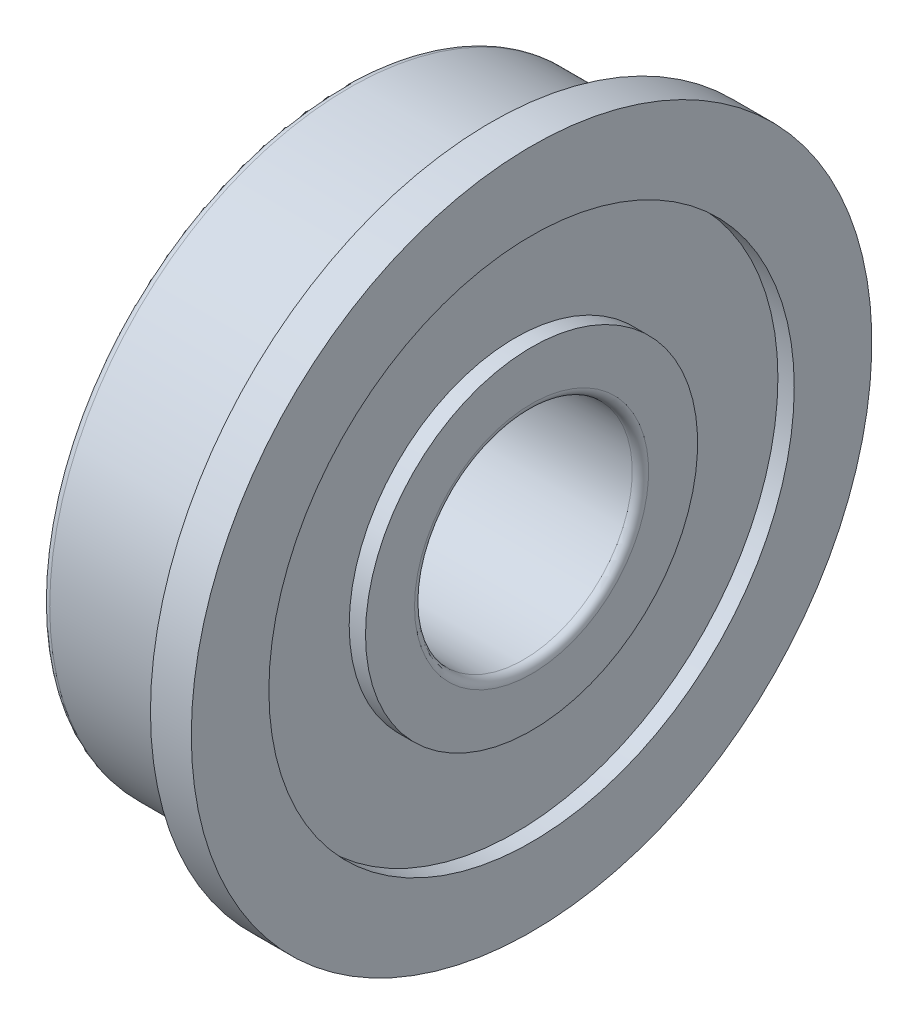
from build123d import *


with BuildPart() as part:
    # Sketch1 → Revolve1 (revolve)
    with BuildSketch(Plane.XY, mode=Mode.PRIVATE) as revolve1_sk:
        with BuildLine():
            Line((0, 10.7), (0, 9.65))
            Line((0, 9.65), (0.6, 9.65))
            Line((0.6, 9.65), (0.6, 6.1))
            Line((0.6, 6.1), (0, 6.1))
            Line((0, 6.1), (0, 4.3))
            ThreePointArc((0, 4.3), (0.087867966, 4.087867966), (0.3, 4))
            Line((0.3, 4), (6.7, 4))
            ThreePointArc((6.7, 4), (6.912132034, 4.087867966), (7, 4.3))
            Line((7, 4.3), (7, 6.1))
            Line((7, 6.1), (6.4, 6.1))
            Line((6.4, 6.1), (6.4, 9.65))
            Line((6.4, 9.65), (7, 9.65))
            Line((7, 9.65), (7, 12.5))
            Line((7, 12.5), (5.5, 12.5))
            Line((5.5, 12.5), (5.5, 11.3))
            ThreePointArc((5.5, 11.3), (5.712132034, 10.787867966), (5.2, 11))
            Line((5.2, 11), (0.3, 11))
            ThreePointArc((0.3, 11), (0.087867966, 10.912132034), (0, 10.7))
        make_face()
    revolve(revolve1_sk.sketch.rotate(Axis((22, 0, 0), (-1, 0, 0)), 270), axis=Axis((22, 0, 0), (-1, 0, 0)))


solid = part.part
